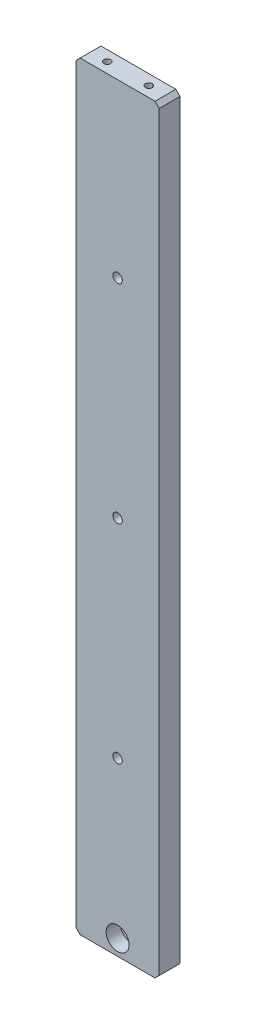
from build123d import *

# Parameters (mm, degrees)
SKETCH1_W                                    = 40
SKETCH1_H                                    = 365
BOSS_EXTRUDE1_DEPTH                          = 5
M4_TAPPED_HOLE2_D                            = 3.3
M4_TAPPED_HOLE2_DEPTH                        = 10.1
M4_TAPPED_HOLE2_TIP                          = 0.991420021
HEX_SOCKET_CAP_SCREW_HOLE_TYPE_1_D           = 6.6
HEX_SOCKET_CAP_SCREW_HOLE_TYPE_1_CBORE_D     = 11
HEX_SOCKET_CAP_SCREW_HOLE_TYPE_1_CBORE_DEPTH = 6.8
M5_TAPPED_HOLE1_D                            = 4.2
M5_TAPPED_HOLE1_DEPTH                        = 14
M5_TAPPED_HOLE1_TIP                          = 1.2618073
CHAMFER1_SIZE                                = 2
HEX_SOCKET_CAP_SCREW_HOLE_TYPE_2_D           = 4.5
HEX_SOCKET_CAP_SCREW_HOLE_TYPE_2_CBORE_D     = 8
HEX_SOCKET_CAP_SCREW_HOLE_TYPE_2_CBORE_DEPTH = 4.6


with BuildPart() as part:
    # Sketch1 → Boss-Extrude1 (new, symmetric)
    with BuildSketch(Plane.XY):
        Rectangle(SKETCH1_W, SKETCH1_H)
    extrude(amount=BOSS_EXTRUDE1_DEPTH, both=True)

    # M4 Tapped Hole2
    with Locations(Plane(origin=(0, 182.5, 0), x_dir=(1, 0, 0), z_dir=(0, 1, 0))):
        with Locations((10, 0), (-10, 0)):
            Hole(M4_TAPPED_HOLE2_D / 2, depth=M4_TAPPED_HOLE2_DEPTH)
            with Locations((0, 0, -(M4_TAPPED_HOLE2_DEPTH + M4_TAPPED_HOLE2_TIP / 2))):  # 118° drill point
                Cone(0, M4_TAPPED_HOLE2_D / 2, M4_TAPPED_HOLE2_TIP, mode=Mode.SUBTRACT)

    # Hex socket cap screw hole type 1 (through all)
    with Locations(Plane.XY.offset(5)):
        with Locations((0, -175)):
            CounterBoreHole(HEX_SOCKET_CAP_SCREW_HOLE_TYPE_1_D / 2, HEX_SOCKET_CAP_SCREW_HOLE_TYPE_1_CBORE_D / 2, HEX_SOCKET_CAP_SCREW_HOLE_TYPE_1_CBORE_DEPTH)

    # M5 Tapped Hole1
    with Locations(Plane.ZY.offset(20)):
        with Locations((0, 0), (0, 100), (0, -100)):
            Hole(M5_TAPPED_HOLE1_D / 2, depth=M5_TAPPED_HOLE1_DEPTH)
            with Locations((0, 0, -(M5_TAPPED_HOLE1_DEPTH + M5_TAPPED_HOLE1_TIP / 2))):  # 118° drill point
                Cone(0, M5_TAPPED_HOLE1_D / 2, M5_TAPPED_HOLE1_TIP, mode=Mode.SUBTRACT)

    # Chamfer1
    chamfer1_edges = [part.edges().sort_by_distance(p)[0] for p in [
        (-20, 182.5, 0),
        (20, 182.5, 0),
        (20, -182.5, 0),
        (-20, -182.5, 0),
    ]]
    chamfer(chamfer1_edges, length=CHAMFER1_SIZE)

    # Hex socket cap screw hole type 2 (through all)
    with Locations(Plane(origin=(0, 0, -5), x_dir=(-1, 0, 0), z_dir=(0, 0, -1))):
        with Locations((0, 100), (0, 0), (0, -100)):
            CounterBoreHole(HEX_SOCKET_CAP_SCREW_HOLE_TYPE_2_D / 2, HEX_SOCKET_CAP_SCREW_HOLE_TYPE_2_CBORE_D / 2, HEX_SOCKET_CAP_SCREW_HOLE_TYPE_2_CBORE_DEPTH)


solid = part.part
